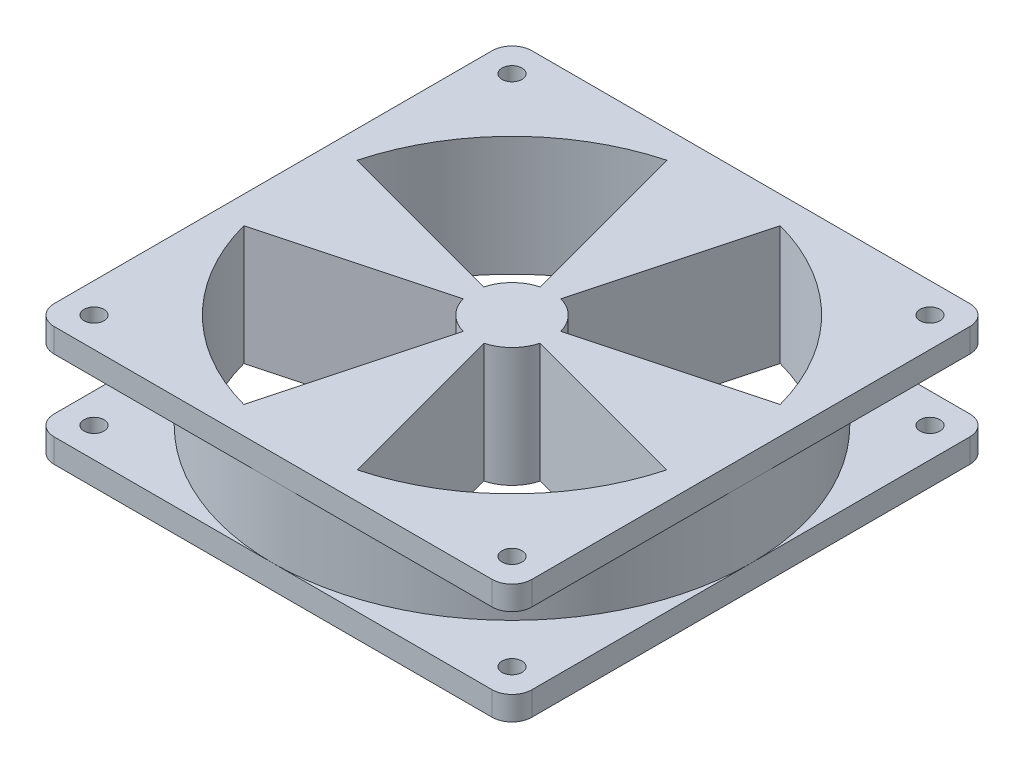
from build123d import *

# Parameters (mm, degrees)
SKETCH_1_W          = 120
SKETCH_1_H          = 120
EXTRUDE_1_DEPTH     = 15
SKETCH_3_R          = 90.791455295
SKETCH_3_R_2        = 60
CUT_EXTRUDE_1_DEPTH = 9
SKETCH_4_R          = 2.5
CUT_EXTRUDE_3_DEPTH = 91
FILLET_1_R          = 5
CUT_EXTRUDE_4_DEPTH = 91


with BuildPart() as part:
    # 草图1 → 凸台-拉伸1 (new, symmetric)
    with BuildSketch(Plane(origin=(0, 0, 0), x_dir=(1, 0, 0), z_dir=(0, 1, 0))):
        Rectangle(SKETCH_1_W, SKETCH_1_H)
    extrude(amount=EXTRUDE_1_DEPTH, both=True)

    # 草图3 → 切除-拉伸1 (cut, symmetric)
    with BuildSketch(Plane(origin=(0, 0, 0), x_dir=(1, 0, 0), z_dir=(0, 1, 0))):
        Circle(SKETCH_3_R)
        with Locations(Location((0, 0, 0), (0, 0, 270))):
            Circle(SKETCH_3_R_2, mode=Mode.SUBTRACT)
    extrude(amount=CUT_EXTRUDE_1_DEPTH, both=True, mode=Mode.SUBTRACT)

    # 草图4 → 切除-拉伸3 (cut, through all)
    with BuildSketch(Plane(origin=(0, 15, 0), x_dir=(1, 0, 0), z_dir=(0, 1, 0))):
        with Locations(Location((-52.5, 52.5, 0), (0, 0, 270))):
            Circle(SKETCH_4_R)
        with Locations(Location((-52.5, -52.5, 0), (0, 0, 270))):
            Circle(SKETCH_4_R)
        with Locations(Location((52.5, -52.5, 0), (0, 0, 270))):
            Circle(SKETCH_4_R)
        with Locations(Location((52.5, 52.5, 0), (0, 0, 270))):
            Circle(SKETCH_4_R)
    extrude(amount=-CUT_EXTRUDE_3_DEPTH, mode=Mode.SUBTRACT)

    # 圆角1
    fillet_1_edges = [part.edges().sort_by_distance(p)[0] for p in [
        (60, -12, 60),
        (-60, -12, 60),
        (-60, -12, -60),
        (60, -12, -60),
        (60, 12, 60),
        (-60, 12, 60),
        (-60, 12, -60),
        (60, 12, -60),
    ]]
    fillet(fillet_1_edges, radius=FILLET_1_R)

    # 草图5 → 切除-拉伸4 (cut, through all)
    with BuildSketch(Plane(origin=(0, 15, 0), x_dir=(1, 0, 0), z_dir=(0, 1, 0))):
        with BuildLine():
            ThreePointArc((-9.659258263, 2.588190451), (-7.071067812, 7.071067812), (-2.588190451, 9.659258263))
            Line((-2.588190451, 9.659258263), (-14.235047481, 53.125920446))
            ThreePointArc((-14.235047481, 53.125920446), (-38.890872965, 38.890872965), (-53.125920446, 14.235047481))
            Line((-53.125920446, 14.235047481), (-9.659258263, 2.588190451))
        make_face()
        with BuildLine():
            Line((14.235047481, 53.125920446), (2.588190451, 9.659258263))
            ThreePointArc((2.588190451, 9.659258263), (7.071067812, 7.071067812), (9.659258263, 2.588190451))
            Line((9.659258263, 2.588190451), (53.125920446, 14.235047481))
            ThreePointArc((53.125920446, 14.235047481), (38.890872965, 38.890872965), (14.235047481, 53.125920446))
        make_face()
        with BuildLine():
            ThreePointArc((9.659258263, -2.588190451), (7.071067812, -7.071067812), (2.588190451, -9.659258263))
            Line((2.588190451, -9.659258263), (14.235047481, -53.125920446))
            ThreePointArc((14.235047481, -53.125920446), (38.890872965, -38.890872965), (53.125920446, -14.235047481))
            Line((53.125920446, -14.235047481), (9.659258263, -2.588190451))
        make_face()
        with BuildLine():
            Line((-14.235047481, -53.125920446), (-2.588190451, -9.659258263))
            ThreePointArc((-2.588190451, -9.659258263), (-7.071067812, -7.071067812), (-9.659258263, -2.588190451))
            Line((-9.659258263, -2.588190451), (-53.125920446, -14.235047481))
            ThreePointArc((-53.125920446, -14.235047481), (-38.890872965, -38.890872965), (-14.235047481, -53.125920446))
        make_face()
    extrude(amount=-CUT_EXTRUDE_4_DEPTH, mode=Mode.SUBTRACT)


solid = part.part
